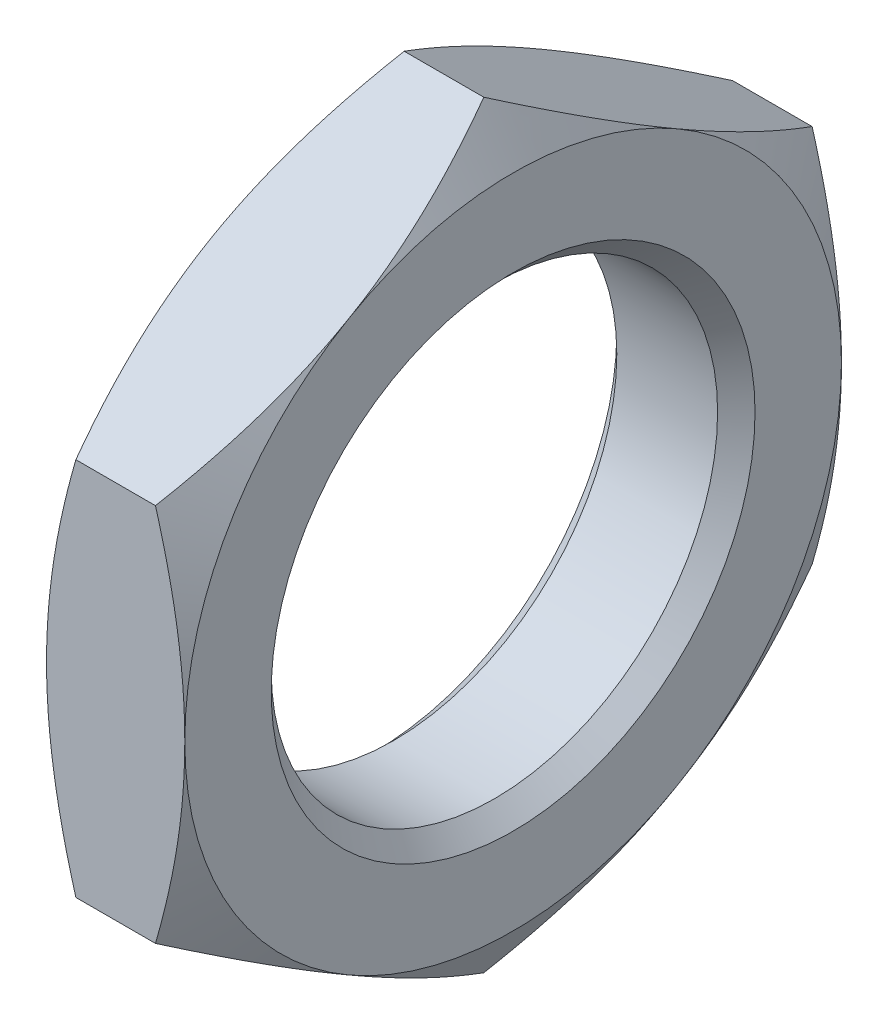
from build123d import *

# Parameters (mm, degrees)
BOSS_EXTRUDE1_DEPTH = 4


with BuildPart() as part:
    # Sketch1 → Boss-Extrude1 (new body)
    with BuildSketch(Plane(origin=(0, 0, 0), x_dir=(0, 0, -1), z_dir=(1, 0, 0))):
        Polygon((-9.5, 5.484827557), (-9.5, -5.484827557), (0, -10.969655115), (9.5, -5.484827557), (9.5, 5.484827557), (0, 10.969655115), align=None)
    extrude(amount=BOSS_EXTRUDE1_DEPTH)

    # Sketch2 → Cut-Revolve1 (revolve, cut)
    with BuildSketch(Plane.XY):
        Polygon((0, 13.95), (0, 9.5), (2, 12.964101615), (4, 9.5), (4, 13.95), align=None)
    revolve(axis=Axis((50, 0, 0), (-1, 0, 0)), mode=Mode.SUBTRACT)

    # Sketch3 → Cut-Revolve2 (revolve, cut)
    with BuildSketch(Plane.XY, mode=Mode.PRIVATE) as cut_revolve2_sk:
        Polygon((0, 0), (0, 7), (0.5415, 6.4585), (3.4585, 6.4585), (4, 7), (4, 0), align=None)
    revolve(cut_revolve2_sk.sketch.rotate(Axis((4, 0, 0), (-1, 0, 0)), 90), axis=Axis((4, 0, 0), (-1, 0, 0)), mode=Mode.SUBTRACT)


solid = part.part
